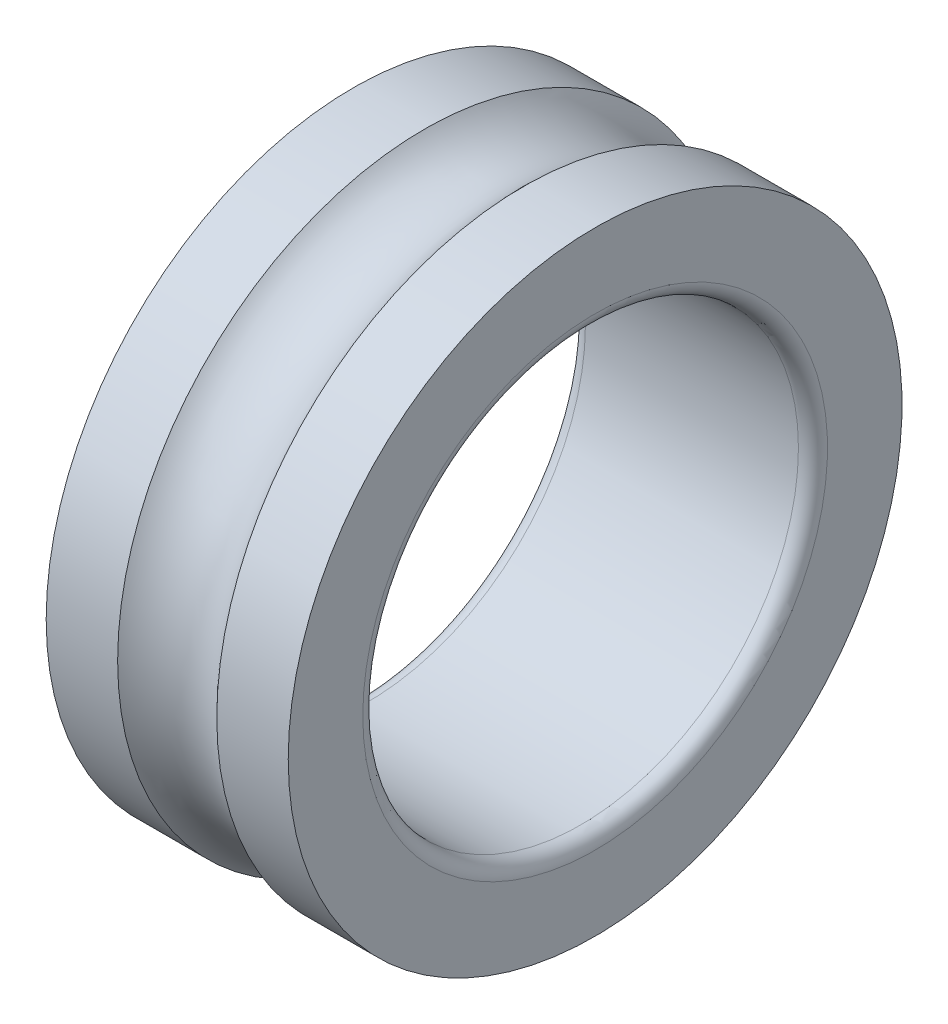
from build123d import *

# Parameters (mm, degrees)
FILLET1_R = 1.5


with BuildPart() as part:
    # Sketch1 → Revolve1 (revolve)
    with BuildSketch(Plane.XY, mode=Mode.PRIVATE) as revolve1_sk:
        with BuildLine():
            Line((5.120546846, 31.7), (12.5, 31.7))
            Line((12.5, 31.7), (12.5, 22.5))
            Line((12.5, 22.5), (-12.5, 22.5))
            Line((-12.5, 22.5), (-12.5, 31.7))
            Line((-12.5, 31.7), (-5.120546846, 31.7))
            ThreePointArc((-5.120546846, 31.7), (0, 29.4), (5.120546846, 31.7))
        make_face()
    revolve(revolve1_sk.sketch.rotate(Axis((-18.919268053, 0, 0), (1, 0, 0)), 90), axis=Axis((-18.919268053, 0, 0), (1, 0, 0)))

    # Fillet1
    fillet1_edges = [part.edges().sort_by_distance(p)[0] for p in [
        (12.5, 0, -22.5),
        (-12.5, 0, -22.5),
    ]]
    fillet(fillet1_edges, radius=FILLET1_R)


solid = part.part
